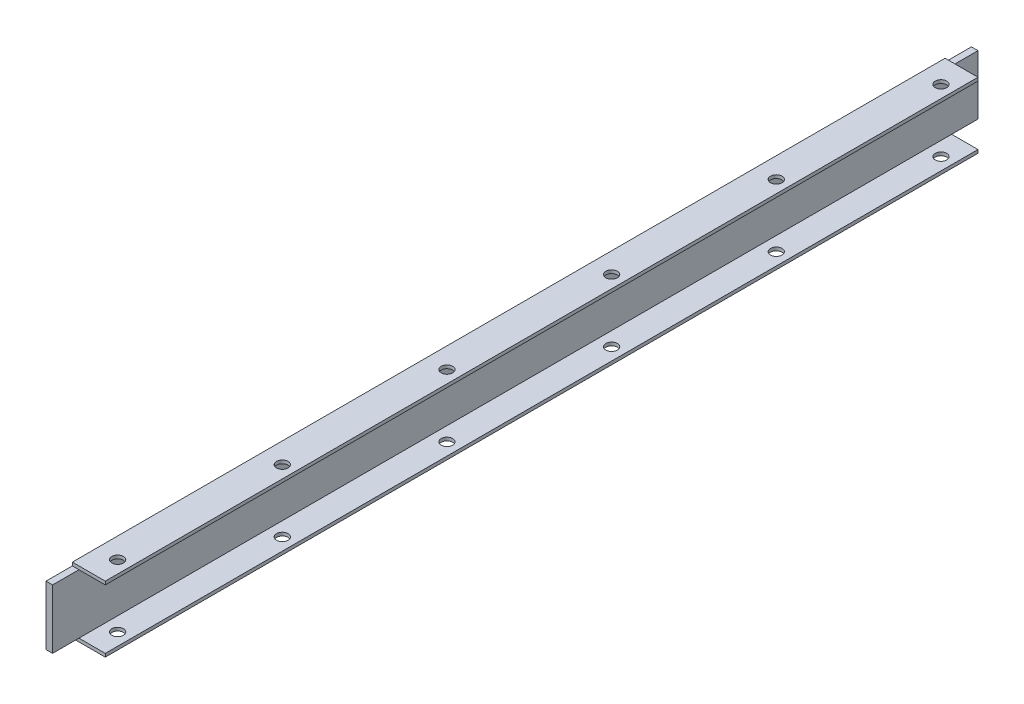
SolidWorks part; units mm, degrees
ref_plane "Front Plane" through (0, 0, 0) normal (0, 0, 1) x (1, 0, 0)
ref_plane "Top Plane" through (0, 0, 0) normal (0, 1, 0) x (1, 0, 0)
ref_plane "Right Plane" through (0, 0, 0) normal (1, 0, 0) x (0, 0, -1)
sketch "Sketch1" plane through (0, 0, 0) normal (0, 0, 1) x (1, 0, 0)
  line L0 (0, 0) -> (-40, 0)
  line L1 (-40, 0) -> (-40, 80)
  line L2 (-40, 80) -> (0, 80)
  line L3 (0, 80) -> (0, 76)
  line L4 (0, 76) -> (-32, 76)
  line L5 (-32, 76) -> (-32, 4)
  line L6 (-32, 4) -> (0, 4)
  line L7 (0, 4) -> (0, 0)
  dimension "D1" = 80
  dimension "D2" = 40
  dimension "D3" = 40
  dimension "D4" = 4
  dimension "D5" = 4
  dimension "D6" = 8
sheet metal parameters "Sheet metal 1" thickness 3 parameters "D1"=3
extrude "Extrude1" add sketch "Sketch1" along normal blind 1124
sketch "Sketch2" plane through (0, 80, 0) normal (0, 1, 0) x (1, 0, 0)
  line L0 (-40, -1124) -> (-40, 0) construction
  line L1 (0, 0) -> (-32, 0)
  line L2 (0, 0) -> (0, -32)
  line L3 (0, -32) -> (-32, -32)
  line L4 (-32, 0) -> (-32, -32)
  line L6 (0, -1124) -> (-32, -1124)
  line L7 (0, -1124) -> (0, -1092)
  line L8 (0, -1092) -> (-32, -1092)
  line L9 (-32, -1124) -> (-32, -1092)
  dimension "D1" = 8
  dimension "D2" = 32
  dimension "D3" = 8
  dimension "D4" = 32
extrude "Cut-Extrude1" cut sketch "Sketch2" against normal through all
sketch "Sketch3" plane through (-32, 0, 0) normal (1, 0, 0) x (0, 0, -1)
  line L1 (-1092, 76) -> (-1124, 76)
  line L2 (-1092, 76) -> (-1092, 80)
  line L3 (-1092, 80) -> (-1124, 80)
  line L4 (-1124, 76) -> (-1124, 80)
  line L5 (-1092, 4) -> (-1124, 4)
  line L6 (-1092, 4) -> (-1092, 0)
  line L7 (-1092, 0) -> (-1124, 0)
  line L8 (-1124, 4) -> (-1124, 0)
  line L9 (-32, 76) -> (0, 76)
  line L10 (-32, 76) -> (-32, 80)
  line L11 (-32, 80) -> (0, 80)
  line L12 (0, 76) -> (0, 80)
  line L14 (-32, 4) -> (0, 4)
  line L15 (-32, 4) -> (-32, 0)
  line L16 (-32, 0) -> (0, 0)
  line L17 (0, 4) -> (0, 0)
extrude "Cut-Extrude2" cut sketch "Sketch3" against normal blind 1200
sketch "Sketch4" plane through (0, 80, 0) normal (0, 1, 0) x (1, 0, 0)
  line L0 (-40, -1092) -> (-40, -32) construction
  line L1 (-40, -1092) -> (-40, -32) construction
  circle A0 centre (-15, -1062) radius 7
  point P2 (-40, -562)
  dimension "D1" = 500
  dimension "D2" = 14
  dimension "D3" = 25
extrude "Cut-Extrude3" cut sketch "Sketch4" against normal through all
pattern_linear "LPattern1" count 6 spacing 200 along (0, 0, -1) of "Cut-Extrude3"
